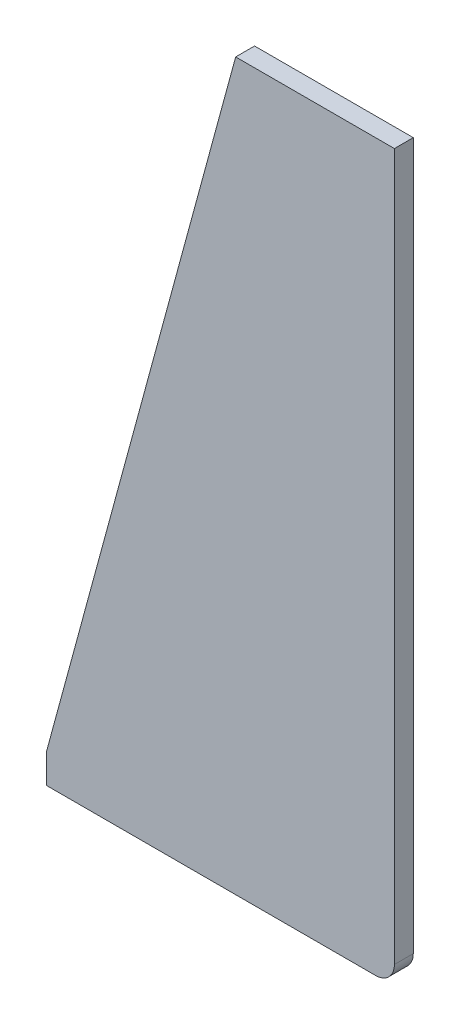
from build123d import *

# Parameters (mm, degrees)
BOSS_EXTRUDE1_DEPTH = 5


with BuildPart() as part:
    # Sketch1 → Boss-Extrude1 (new body)
    with BuildSketch(Plane.XY):
        with BuildLine():
            Line((0, 0), (-50, -184))
            Line((-50, -184), (-50, -192))
            Line((-50, -192), (37, -192))
            ThreePointArc((37, -192), (40.535533906, -190.535533906), (42, -187))
            Line((42, -187), (42, 0))
            Line((42, 0), (0, 0))
        make_face()
    extrude(amount=BOSS_EXTRUDE1_DEPTH)


solid = part.part
